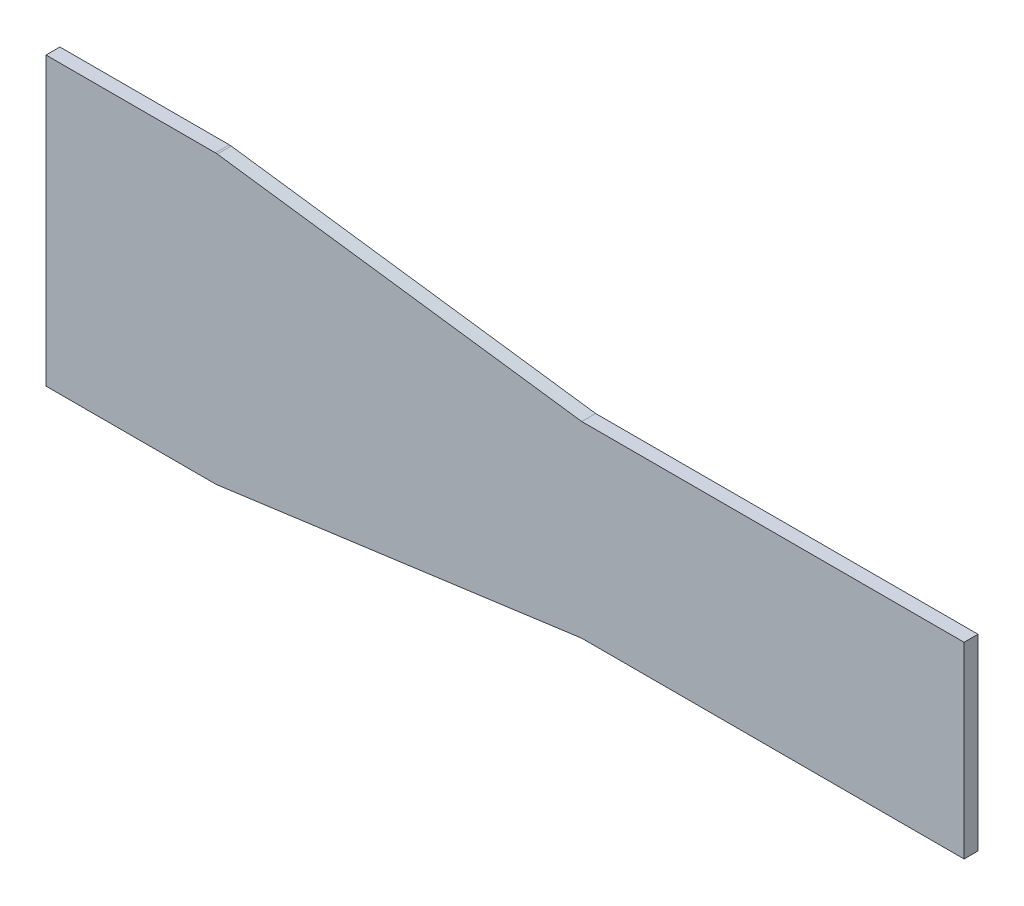
SolidWorks part; units mm, degrees
ref_plane "Front Plane" through (0, 0, 0) normal (0, 0, 1) x (1, 0, 0)
ref_plane "Top Plane" through (0, 0, 0) normal (0, 1, 0) x (1, 0, 0)
ref_plane "Right Plane" through (0, 0, 0) normal (1, 0, 0) x (0, 0, -1)
sketch "Sketch1" plane through (0, 0, 0) normal (0, 0, 1) x (1, 0, 0)
  line L0 (0, 0) -> (1274.8609, 0) construction
  line L1 (0, 165) -> (194.9205, 165)
  line L2 (0, -165) -> (0, 165)
  line L3 (1056.5, 108) -> (1056.5, -108)
  line L4 (1056.5, 108) -> (616.5, 108)
  line L5 (616.5, 108) -> (197.0697, 164.855)
  line L6 (1056.5, -108) -> (616.5, -108)
  line L7 (616.5, -108) -> (197.0697, -164.855)
  line L8 (0, -165) -> (194.9205, -165)
  arc A0 (194.9205, 165) -> (197.0697, 164.855) centre (194.9205, 149) cw
  arc A1 (194.9205, -165) -> (197.0697, -164.855) centre (194.9205, -149) ccw
  point P10 (196, 165)
  point P12 (1056.5, 0)
  point P16 (196, -165)
  dimension "D6" = 16
  dimension "D1" = 196
  dimension "D2" = 330
  dimension "D3" = 1056.5
  dimension "D4" = 216
  dimension "D5" = 440
extrude "Boss-Extrude1" add sketch "Sketch1" along normal blind 16
